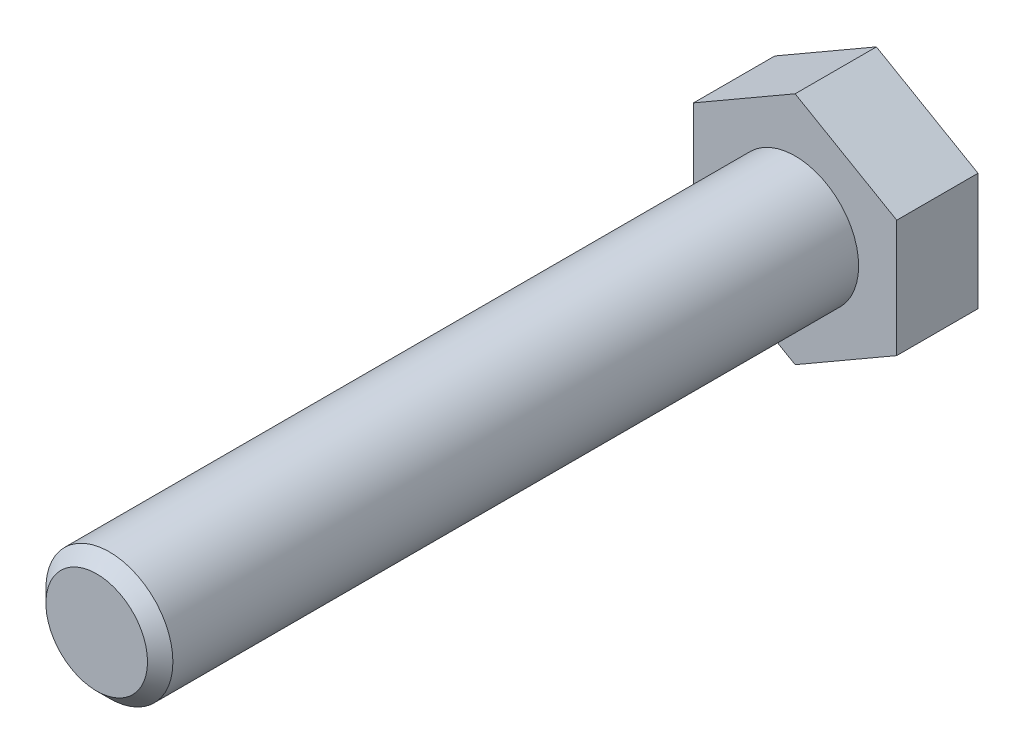
from build123d import *

# Parameters (mm, degrees)
BOSS_EXTRUDE1_DEPTH = 6.4
SKETCH3_R           = 5
BOSS_EXTRUDE2_DEPTH = 55
CHAMFER1_SIZE       = 1


with BuildPart() as part:
    # Sketch1 → Boss-Extrude1 (new body)
    with BuildSketch(Plane.XY):
        Polygon((8, 4.618802154), (0, 9.237604307), (-8, 4.618802154), (-8, -4.618802154), (0, -9.237604307), (8, -4.618802154), align=None)
    extrude(amount=BOSS_EXTRUDE1_DEPTH)

    # Sketch3 → Boss-Extrude2 (add)
    with BuildSketch(Plane.XY.offset(6.4)):
        Circle(SKETCH3_R)
    extrude(amount=BOSS_EXTRUDE2_DEPTH)

    # Chamfer1
    chamfer1_edges = [part.edges().sort_by_distance(p)[0] for p in [
        (-5, 0, 61.4),
    ]]
    chamfer(chamfer1_edges, length=CHAMFER1_SIZE)


solid = part.part
